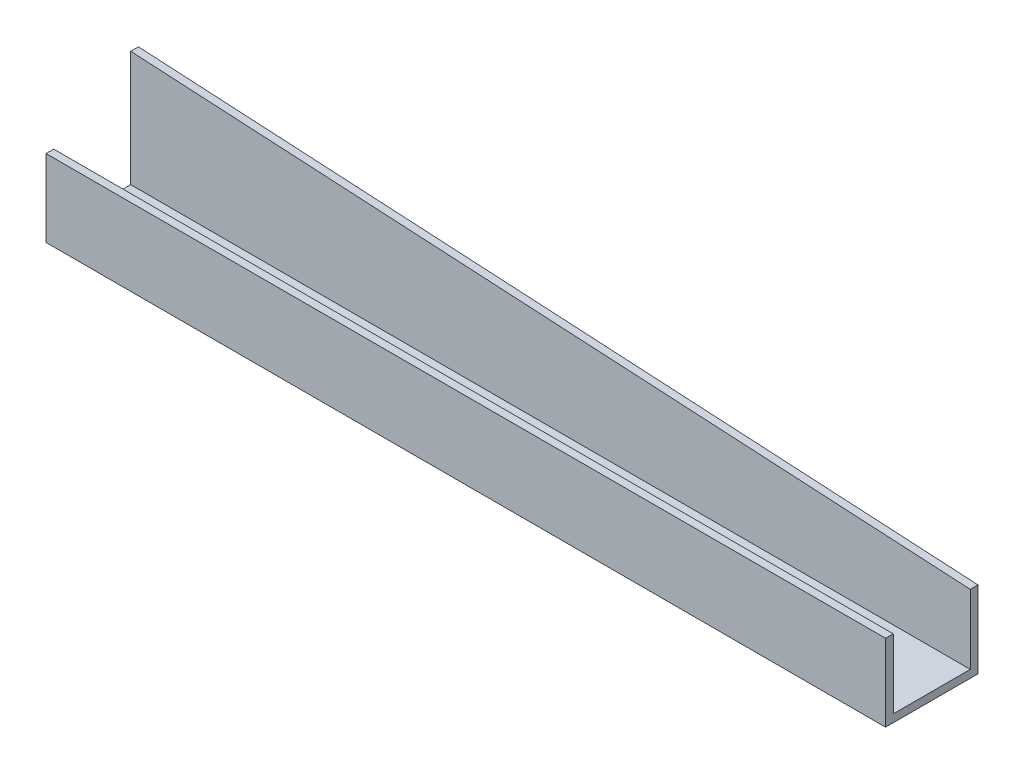
SolidWorks part; units mm, degrees
ref_plane "前视基准面" through (0, 0, 0) normal (0, 0, 1) x (1, 0, 0)
ref_plane "上视基准面" through (0, 0, 0) normal (0, 1, 0) x (1, 0, 0)
ref_plane "右视基准面" through (0, 0, 0) normal (1, 0, 0) x (0, 0, -1)
sketch "草图1" plane through (0, 0, 0) normal (0, 0, 1) x (1, 0, 0)
  line L0 (0, 0) -> (0, -80)
  line L1 (545, -80) -> (545, -30)
  line L2 (545, -30) -> (0, 0)
  line L3 (0, -80) -> (545, -80)
extrude "凸台-拉伸1" add sketch "草图1" along normal blind 60
shell "抽壳2" thickness 5
sketch "草图4" plane through (0, 0, 60) normal (0, 0, 1) x (1, 0, 0)
  line L0 (545, -30) -> (0, -30)
  line L1 (0, 0) -> (0, -80) construction
  line L2 (0, -30) -> (0, 50.0344)
  line L3 (0, 50.0344) -> (545, -30)
extrude "切除-拉伸2" cut sketch "草图4" against normal blind 38
